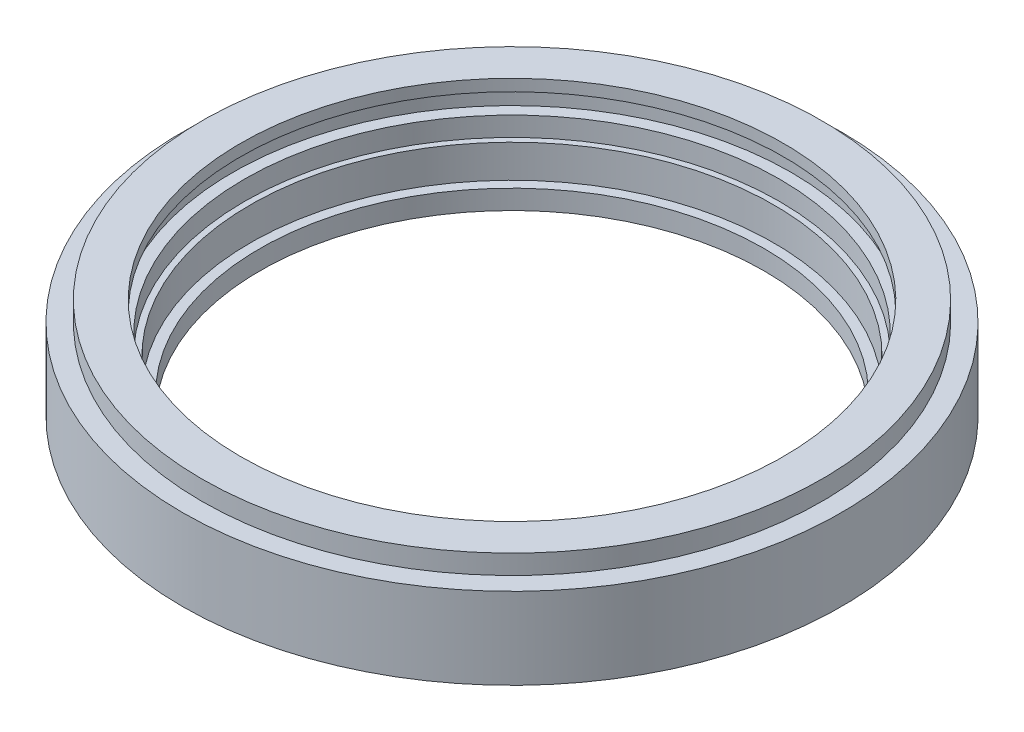
SolidWorks part; units mm, degrees
material "Q235"
ref_plane "Front Plane" through (0, 0, 0) normal (0, 0, 1) x (1, 0, 0)
ref_plane "Top Plane" through (0, 0, 0) normal (0, 1, 0) x (1, 0, 0)
ref_plane "Right Plane" through (0, 0, 0) normal (1, 0, 0) x (0, 0, -1)
sketch "Sketch1" plane through (0, 0, 0) normal (0, 0, 1) x (1, 0, 0)
  line L0 (70, 0) -> (80, 0)
  line L1 (80, 0) -> (80, -5)
  line L2 (80, -5) -> (85, -5)
  line L3 (85, -5) -> (85, -26)
  line L4 (85, -26) -> (65, -26)
  line L5 (65, -26) -> (65, -21)
  line L6 (65, -21) -> (67.5, -21)
  line L7 (69, -12.5) -> (69, -7.5)
  line L8 (69, -7.5) -> (72, -7.5)
  line L9 (72, -7.5) -> (72, -3)
  line L10 (72, -3) -> (70, -3)
  line L11 (70, -3) -> (70, 0)
  line L12 (69, -12.5) -> (67.5, -12.5)
  line L13 (67.5, -12.5) -> (67.5, -21)
  line L14 (0, 0) -> (0, -22.1185) construction
  dimension "D1" = 67.5
  dimension "D2" = 65
  dimension "D3" = 5
  dimension "D4" = 26
  dimension "D5" = 69
  dimension "D6" = 5
  dimension "D7" = 4.5
  dimension "D8" = 72
  dimension "D9" = 3
  dimension "D10" = 85
  dimension "D11" = 80
  dimension "D12" = 5
  dimension "D13" = 70
revolve "Revolve1" add sketch "Sketch1" angle 360 about L14
